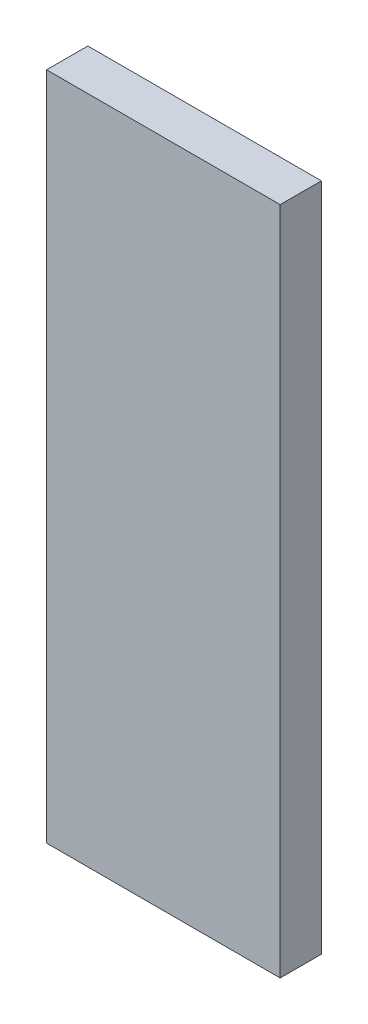
from build123d import *

# Parameters (mm, degrees)
SKETCH1_W           = 68
SKETCH1_H           = 195
BOSS_EXTRUDE1_DEPTH = 12


with BuildPart() as part:
    # Sketch1 → Boss-Extrude1 (new body)
    with BuildSketch(Plane.XY):
        with Locations((34, 97.5)):
            Rectangle(SKETCH1_W, SKETCH1_H)
    extrude(amount=BOSS_EXTRUDE1_DEPTH)


solid = part.part
